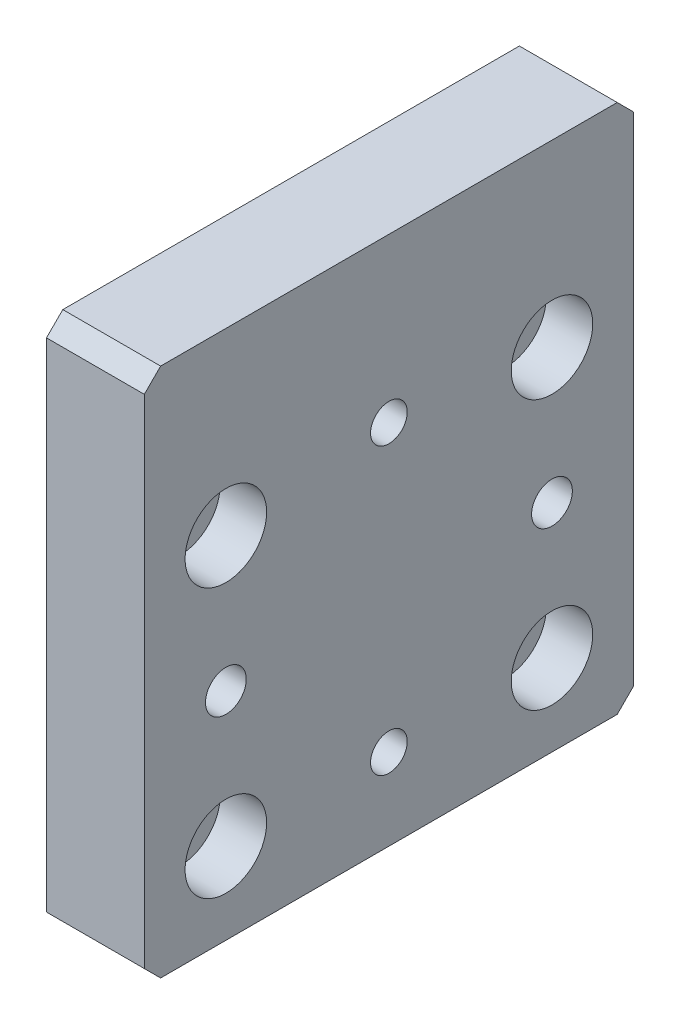
SolidWorks part; units mm, degrees
material "AL6061"
ref_plane "Front Plane" through (0, 0, 0) normal (0, 0, 1) x (1, 0, 0)
ref_plane "Top Plane" through (0, 0, 0) normal (0, 1, 0) x (1, 0, 0)
ref_plane "Right Plane" through (0, 0, 0) normal (1, 0, 0) x (0, 0, -1)
sketch "Sketch1" plane through (0, 0, 0) normal (1, 0, 0) x (0, 0, -1)
  line L1 (-30, -32.5) -> (30, -32.5)
  line L2 (-30, -32.5) -> (-30, 32.5)
  line L3 (-30, 32.5) -> (30, 32.5)
  line L4 (30, -32.5) -> (30, 32.5)
  line L5 (-30, -32.5) -> (30, 32.5) construction
  line L6 (-30, 32.5) -> (30, -32.5) construction
  point P0 (0, 0)
  dimension "D1" = 60
  dimension "D2" = 65
extrude "Boss-Extrude1" add sketch "Sketch1" along normal blind 12
hole_wizard "CBORE for M4 Hexagon socket head cap screws1" positions "Sketch2" profile "Sketch3" counterbore size "M4" standard "GB" end condition through all
sketch "Sketch2" plane through (0, 0, 0) normal (-1, 0, 0) x (0, 0, 1)
  line L3 (30, -32.5) -> (-30, -32.5) construction
  point P0 (0, 12.5)
  point P2 (0, -22.5)
  dimension "D1" = 35
  dimension "D2" = 10
sketch "Sketch3" plane through (0, 12.5, 0) normal (0, 1, 0) x (0, 0, 1)
  line L0 (0, 0) -> (0, 12)
  line L1 (0, 12) -> (2.25, 12)
  line L3 (2.25, 12) -> (2.25, 4.6)
  line L4 (2.25, 4.6) -> (4, 4.6)
  line L5 (4, 4.6) -> (4, 0)
  line L7 (4, 0) -> (0, 0)
  line L11 (0, -6.35) -> (0, 107.95) construction
  dimension "通孔孔直径" = 4.5
  dimension "通孔孔深度" = 12
  dimension "柱形沉头孔直径" = 8
  dimension "柱形沉头孔深度" = 4.6
hole_wizard "CBORE for M5 Hexagon socket head cap screws1" positions "Sketch4" profile "Sketch5" counterbore size "M5" standard "GB" end condition through all
sketch "Sketch4" plane through (12, 0, 0) normal (1, 0, 0) x (0, 0, -1)
  line L0 (0, 32.5) -> (0, 0) construction
  line L1 (30, 32.5) -> (-30, 32.5) construction
  line L3 (-30, -32.5) -> (30, -32.5) construction
  point P0 (-20, 10.5)
  point P2 (-20, -22.5)
  point P12 (20, -22.5)
  point P13 (20, 10.5)
  dimension "D1" = 10
  dimension "D2" = 33
  dimension "D3" = 40
sketch "Sketch5" plane through (12, 10.5, 20) normal (0, 1, 0) x (0, 0, -1)
  line L0 (0, 0) -> (0, 12)
  line L1 (0, 12) -> (2.75, 12)
  line L3 (2.75, 12) -> (2.75, 5.7)
  line L4 (2.75, 5.7) -> (5, 5.7)
  line L5 (5, 5.7) -> (5, 0)
  line L7 (5, 0) -> (0, 0)
  line L11 (0, -6.35) -> (0, 107.95) construction
  dimension "通孔孔直径" = 5.5
  dimension "通孔孔深度" = 12
  dimension "柱形沉头孔直径" = 10
  dimension "柱形沉头孔深度" = 5.7
chamfer "Chamfer1" distance 2 angle 45 4 edges at (6, -32.5, 30) (6, -32.5, -30) (6, 32.5, 30) (6, 32.5, -30)
hole_wizard "Ø5.0mm blind dowel hole1" positions "Sketch6" profile "Sketch7" hole size "Ø5.0" standard "GB" end condition through all
sketch "Sketch6" plane through (12, 0, 0) normal (1, 0, 0) x (0, 0, -1)
  line L0 (-20, 10.5) -> (-20, -22.5) construction
  line L2 (20, 10.5) -> (20, -22.5) construction
  point P13 (20, -6)
  point P16 (-20, -6)
sketch "Sketch7" plane through (12, -6, 20) normal (0, 1, 0) x (0, 0, -1)
  line L0 (0, 0) -> (0, 12)
  line L1 (0, 12) -> (2.5, 12)
  line L2 (2.5, 12) -> (2.5, 0)
  line L5 (2.5, 0) -> (0, 0)
  line L11 (0, -6.35) -> (0, 107.95) construction
  dimension "通孔孔直径" = 5
  dimension "通孔孔深度" = 12
